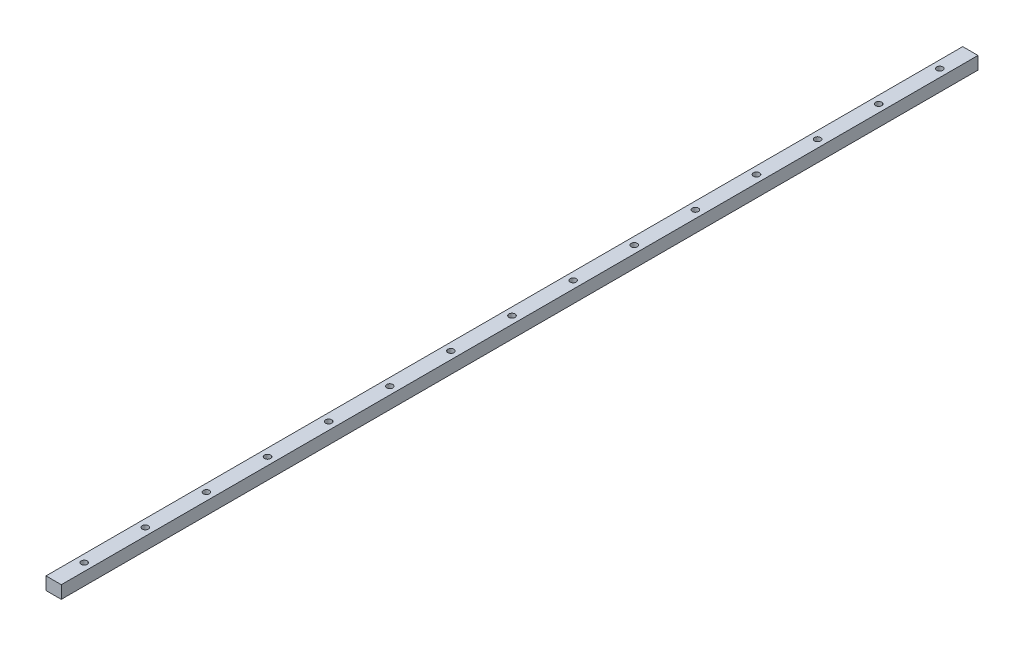
from build123d import *

# Parameters (mm, degrees)
SKETCH_1_W             = 15
SKETCH_1_H             = 12.5
EXTRUDE_1_DEPTH        = 450
SKETCH_2_R             = 3
CUT_EXTRUDE_1_DEPTH    = 4.5
SKETCH_3_R             = 2.25
CUT_EXTRUDE_2_DEPTH    = 451.236049201
PATTERN_LINEAR_1_COUNT = 16
PATTERN_LINEAR_1_PITCH = 60


with BuildPart() as part:
    # 草图1 → 凸台-拉伸1 (new, symmetric)
    with BuildSketch(Plane.XY):
        Rectangle(SKETCH_1_W, SKETCH_1_H)
    extrude(amount=EXTRUDE_1_DEPTH, both=True)

    # 草图2 → 切除-拉伸1 (cut)
    with BuildSketch(Plane(origin=(0, 6.25, 0), x_dir=(1, 0, 0), z_dir=(0, 1, 0))):
        with Locations(Location((0, -420, 0), (0, 0, 270))):
            Circle(SKETCH_2_R)
    cut_extrude_1 = extrude(amount=-CUT_EXTRUDE_1_DEPTH, mode=Mode.SUBTRACT)

    # 草图3 → 切除-拉伸2 (cut, through all)
    with BuildSketch(Plane(origin=(0, 6.25, 0), x_dir=(1, 0, 0), z_dir=(0, 1, 0))):
        with Locations(Location((0, -420, 0), (0, 0, 270))):
            Circle(SKETCH_3_R)
    cut_extrude_2 = extrude(amount=-CUT_EXTRUDE_2_DEPTH, mode=Mode.SUBTRACT)

    # 阵列(线性)1: 切除-拉伸1, 切除-拉伸2 ×16
    with Locations(*[(0, 0, -i * PATTERN_LINEAR_1_PITCH) for i in range(1, PATTERN_LINEAR_1_COUNT)]):
        add(cut_extrude_1, mode=Mode.SUBTRACT)
        add(cut_extrude_2, mode=Mode.SUBTRACT)


solid = part.part
